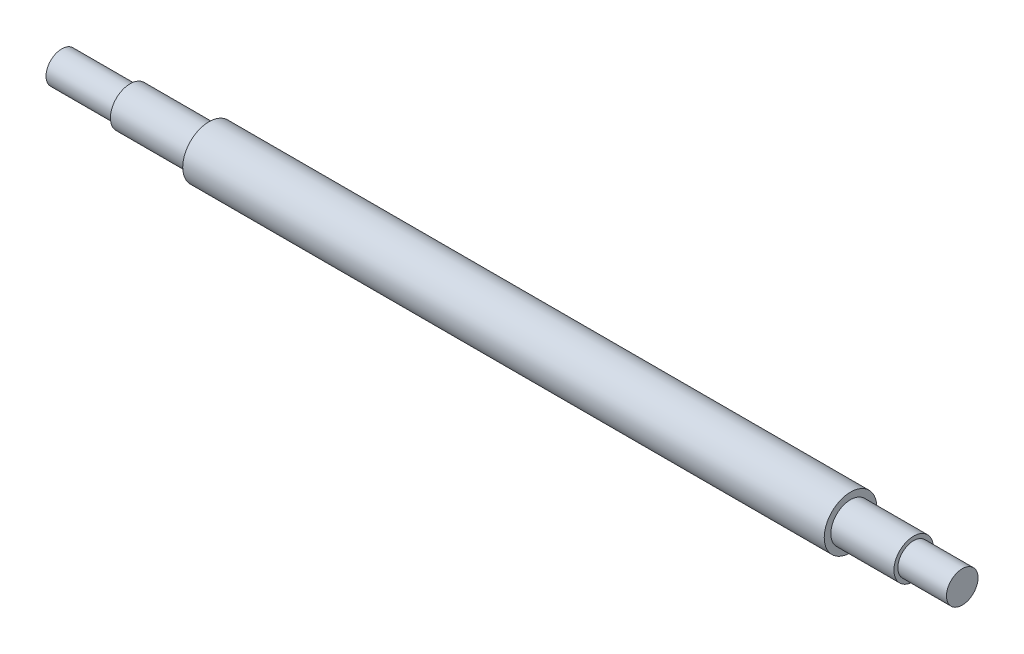
SolidWorks part; units mm, degrees
ref_plane "前视基准面" through (0, 0, 0) normal (0, 0, 1) x (1, 0, 0)
ref_plane "上视基准面" through (0, 0, 0) normal (0, 1, 0) x (1, 0, 0)
ref_plane "右视基准面" through (0, 0, 0) normal (1, 0, 0) x (0, 0, -1)
sketch "草图1" plane through (0, 0, 0) normal (0, 0, 1) x (1, 0, 0)
  line L0 (-124.9032, 0) -> (139.0968, 0) construction
  line L1 (-94.7097, 0) -> (-94.7097, 12)
  line L2 (-94.7097, 12) -> (-42.7097, 12)
  line L3 (-42.7097, 12) -> (-42.7097, 15)
  line L4 (-42.7097, 15) -> (17.2903, 15)
  line L5 (17.2903, 15) -> (17.2903, 20)
  line L6 (17.2903, 20) -> (505.2903, 20)
  line L7 (505.2903, 20) -> (505.2903, 15)
  line L8 (505.2903, 15) -> (553.2903, 15)
  line L9 (553.2903, 15) -> (553.2903, 12)
  line L10 (553.2903, 12) -> (590.2903, 12)
  line L11 (590.2903, 12) -> (590.2903, 0)
  line L12 (590.2903, 0) -> (-94.7097, 0)
  dimension "D1" = 12
  dimension "D2" = 3
  dimension "D3" = 5
  dimension "D4" = 5
  dimension "D5" = 3
  dimension "D6" = 52
  dimension "D7" = 37
  dimension "D8" = 48
  dimension "D9" = 488
  dimension "D10" = 60
revolve "旋转1" add sketch "草图1" angle 360 about L0
cosmetic thread "装饰螺纹线1"
cosmetic thread "装饰螺纹线2"
cosmetic thread "装饰螺纹线3"
